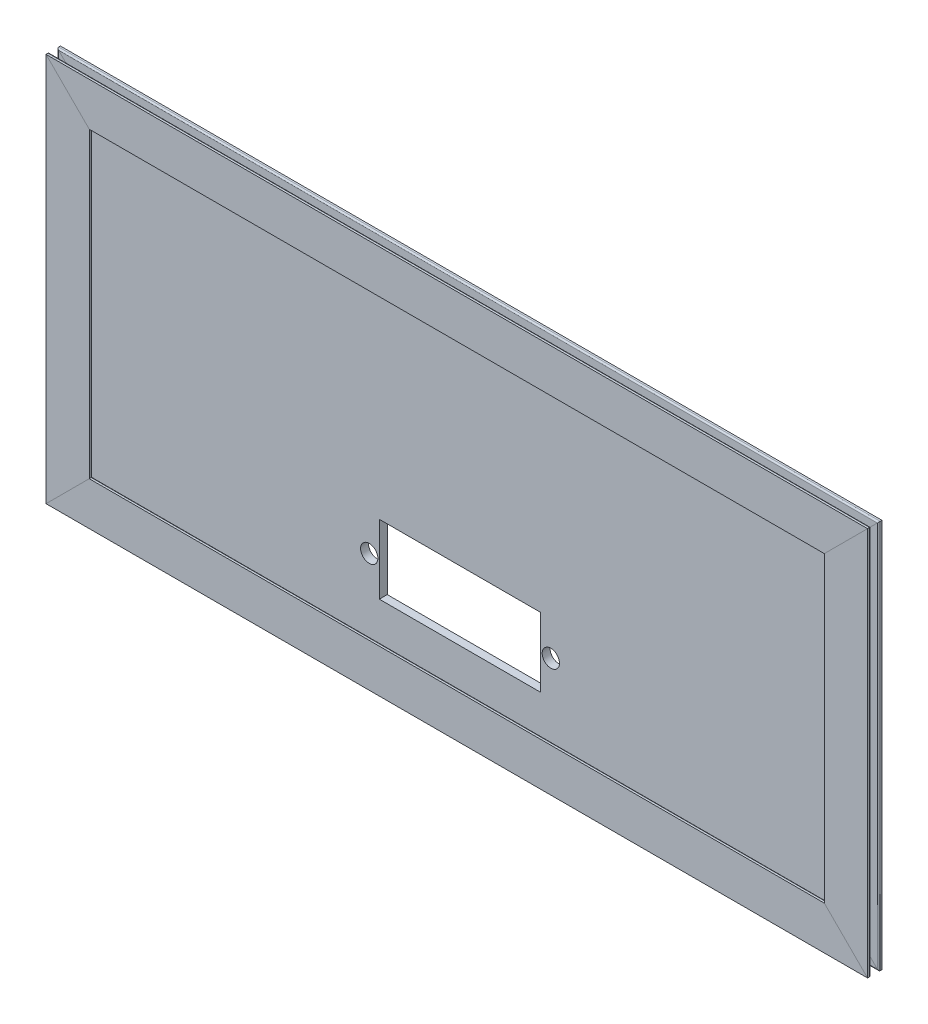
from build123d import *

# Parameters (mm, degrees)
ALUMINIUM_PROFILE_20_X_20_X_2_1_DEPTH      = 556.811388301
ALUMINIUM_PROFILE_20_X_20_X_2_1_DEPTH_BACK = 16.811388301
SKETCH1_W                                  = 6.2
SKETCH1_H                                  = 4.4
SKETCH1_ON_SEGMENT_2_W                     = 6.2
SKETCH1_ON_SEGMENT_2_H                     = 4.4
ALUMINIUM_PROFILE_20_X_20_X_2_1_2_DEPTH    = 273.622776602
SKETCH1_ON_SEGMENT_3_W                     = 6.2
SKETCH1_ON_SEGMENT_3_H                     = 4.4
ALUMINIUM_PROFILE_20_X_20_X_2_1_3_DEPTH    = 573.622776602
SKETCH1_ON_SEGMENT_4_W                     = 6.2
SKETCH1_ON_SEGMENT_4_H                     = 4.4
ALUMINIUM_PROFILE_20_X_20_X_2_1_4_DEPTH    = 273.622776602
SKETCH3_W                                  = 512
SKETCH3_H                                  = 212
BOSS_EXTRUDE1_DEPTH                        = 5.5
SKETCH4_R                                  = 6
SKETCH4_W                                  = 112
SKETCH4_H                                  = 48
CUT_EXTRUDE1_DEPTH                         = 316.452155643


with BuildPart() as part:
    # Sketch1 → Aluminium profile 20 X 20 X 2(1) (new, two sides: drawn at the far end of the back side and taken through both)
    with BuildSketch(Plane(origin=(-270, 120, 0), x_dir=(0, 1, 0), z_dir=(1, 0, 0)).offset(-ALUMINIUM_PROFILE_20_X_20_X_2_1_DEPTH_BACK)):
        with BuildLine():
            Line((4.5, 2.75), (14, 2.75))
            ThreePointArc((14, 2.75), (14.707106781, 3.042893219), (15, 3.75))
            Line((15, 3.75), (15, 5))
            Line((15, 5), (-15, 5))
            Line((-15, 5), (-15, 3.75))
            ThreePointArc((-15, 3.75), (-14.707106781, 3.042893219), (-14, 2.75))
            Line((-14, 2.75), (-4.5, 2.75))
            Line((-4.5, 2.75), (-4.5, -2.75))
            Line((-4.5, -2.75), (-14, -2.75))
            ThreePointArc((-14, -2.75), (-14.707106781, -3.042893219), (-15, -3.75))
            Line((-15, -3.75), (-15, -5))
            Line((-15, -5), (15, -5))
            Line((15, -5), (15, -3.75))
            ThreePointArc((15, -3.75), (14.707106781, -3.042893219), (14, -2.75))
            Line((14, -2.75), (4.5, -2.75))
            Line((4.5, -2.75), (4.5, 2.75))
        make_face()
        Rectangle(SKETCH1_W, SKETCH1_H, mode=Mode.SUBTRACT)
    extrude(amount=ALUMINIUM_PROFILE_20_X_20_X_2_1_DEPTH + ALUMINIUM_PROFILE_20_X_20_X_2_1_DEPTH_BACK)

    # Aluminium profile 20 X 20 X 2(1) mitre 1
    split(bisect_by=Plane(origin=(-270, 120, 0), x_dir=(-0.707106781, 0.707106781, 0), z_dir=(0.707106781, 0.707106781, 0)), keep=Keep.TOP)

    # Aluminium profile 20 X 20 X 2(1) mitre 2
    split(bisect_by=Plane(origin=(270, 120, 0), x_dir=(-0.707106781, -0.707106781, 0), z_dir=(-0.707106781, 0.707106781, 0)), keep=Keep.TOP)


with BuildPart() as body_2:
    # Sketch1 on segment 2 (carried to segment 2) → Aluminium profile 20 X 20 X 2_1 2 (new body)
    with BuildSketch(Plane(origin=(270, 136.811388301, 0), x_dir=(1, 0, 0), z_dir=(0, -1, 0))):
        with BuildLine():
            Line((4.5, 2.75), (14, 2.75))
            ThreePointArc((14, 2.75), (14.707106781, 3.042893219), (15, 3.75))
            Line((15, 3.75), (15, 5))
            Line((15, 5), (-15, 5))
            Line((-15, 5), (-15, 3.75))
            ThreePointArc((-15, 3.75), (-14.707106781, 3.042893219), (-14, 2.75))
            Line((-14, 2.75), (-4.5, 2.75))
            Line((-4.5, 2.75), (-4.5, -2.75))
            Line((-4.5, -2.75), (-14, -2.75))
            ThreePointArc((-14, -2.75), (-14.707106781, -3.042893219), (-15, -3.75))
            Line((-15, -3.75), (-15, -5))
            Line((-15, -5), (15, -5))
            Line((15, -5), (15, -3.75))
            ThreePointArc((15, -3.75), (14.707106781, -3.042893219), (14, -2.75))
            Line((14, -2.75), (4.5, -2.75))
            Line((4.5, -2.75), (4.5, 2.75))
        make_face()
        Rectangle(SKETCH1_ON_SEGMENT_2_W, SKETCH1_ON_SEGMENT_2_H, mode=Mode.SUBTRACT)
    extrude(amount=ALUMINIUM_PROFILE_20_X_20_X_2_1_2_DEPTH)

    # Aluminium profile 20 X 20 X 2_1 2 mitre
    split(bisect_by=Plane(origin=(270, -120, 0), x_dir=(-0.707106781, 0.707106781, 0), z_dir=(0.707106781, 0.707106781, 0)), keep=Keep.TOP)

    # Aluminium profile 20 X 20 X 2_1 2 mi 2
    split(bisect_by=Plane(origin=(270, 120, 0), x_dir=(0.707106781, 0.707106781, 0), z_dir=(0.707106781, -0.707106781, 0)), keep=Keep.TOP)


with BuildPart() as body_3:
    # Sketch1 on segment 3 (carried to segment 3) → Aluminium profile 20 X 20 X 2_1 3 (new body)
    with BuildSketch(Plane(origin=(286.811388301, -120, 0), x_dir=(0, -1, 0), z_dir=(-1, 0, 0))):
        with BuildLine():
            Line((4.5, 2.75), (14, 2.75))
            ThreePointArc((14, 2.75), (14.707106781, 3.042893219), (15, 3.75))
            Line((15, 3.75), (15, 5))
            Line((15, 5), (-15, 5))
            Line((-15, 5), (-15, 3.75))
            ThreePointArc((-15, 3.75), (-14.707106781, 3.042893219), (-14, 2.75))
            Line((-14, 2.75), (-4.5, 2.75))
            Line((-4.5, 2.75), (-4.5, -2.75))
            Line((-4.5, -2.75), (-14, -2.75))
            ThreePointArc((-14, -2.75), (-14.707106781, -3.042893219), (-15, -3.75))
            Line((-15, -3.75), (-15, -5))
            Line((-15, -5), (15, -5))
            Line((15, -5), (15, -3.75))
            ThreePointArc((15, -3.75), (14.707106781, -3.042893219), (14, -2.75))
            Line((14, -2.75), (4.5, -2.75))
            Line((4.5, -2.75), (4.5, 2.75))
        make_face()
        Rectangle(SKETCH1_ON_SEGMENT_3_W, SKETCH1_ON_SEGMENT_3_H, mode=Mode.SUBTRACT)
    extrude(amount=ALUMINIUM_PROFILE_20_X_20_X_2_1_3_DEPTH)

    # Aluminium profile 20 X 20 X 2_1 3 mitre
    split(bisect_by=Plane(origin=(-270, -120, 0), x_dir=(0.707106781, 0.707106781, 0), z_dir=(0.707106781, -0.707106781, 0)), keep=Keep.TOP)

    # Aluminium profile 20 X 20 X 2_1 3 mi 2
    split(bisect_by=Plane(origin=(270, -120, 0), x_dir=(0.707106781, -0.707106781, 0), z_dir=(-0.707106781, -0.707106781, 0)), keep=Keep.TOP)


with BuildPart() as body_4:
    # Sketch1 on segment 4 (carried to segment 4) → Aluminium profile 20 X 20 X 2_1 4 (new body)
    with BuildSketch(Plane(origin=(-270, -136.811388301, 0), x_dir=(-1, 0, 0), z_dir=(0, 1, 0))):
        with BuildLine():
            Line((4.5, 2.75), (14, 2.75))
            ThreePointArc((14, 2.75), (14.707106781, 3.042893219), (15, 3.75))
            Line((15, 3.75), (15, 5))
            Line((15, 5), (-15, 5))
            Line((-15, 5), (-15, 3.75))
            ThreePointArc((-15, 3.75), (-14.707106781, 3.042893219), (-14, 2.75))
            Line((-14, 2.75), (-4.5, 2.75))
            Line((-4.5, 2.75), (-4.5, -2.75))
            Line((-4.5, -2.75), (-14, -2.75))
            ThreePointArc((-14, -2.75), (-14.707106781, -3.042893219), (-15, -3.75))
            Line((-15, -3.75), (-15, -5))
            Line((-15, -5), (15, -5))
            Line((15, -5), (15, -3.75))
            ThreePointArc((15, -3.75), (14.707106781, -3.042893219), (14, -2.75))
            Line((14, -2.75), (4.5, -2.75))
            Line((4.5, -2.75), (4.5, 2.75))
        make_face()
        Rectangle(SKETCH1_ON_SEGMENT_4_W, SKETCH1_ON_SEGMENT_4_H, mode=Mode.SUBTRACT)
    extrude(amount=ALUMINIUM_PROFILE_20_X_20_X_2_1_4_DEPTH)

    # Aluminium profile 20 X 20 X 2_1 4 mitre
    split(bisect_by=Plane(origin=(-270, -120, 0), x_dir=(-0.707106781, -0.707106781, 0), z_dir=(-0.707106781, 0.707106781, 0)), keep=Keep.TOP)

    # Aluminium profile 20 X 20 X 2_1 4 mi 2
    split(bisect_by=Plane(origin=(-270, 120, 0), x_dir=(0.707106781, -0.707106781, 0), z_dir=(-0.707106781, -0.707106781, 0)), keep=Keep.TOP)


with BuildPart() as body_5:
    # Sketch3 → Boss-Extrude1 (new body)
    with BuildSketch(Plane.XY.offset(-2.75)):
        Rectangle(SKETCH3_W, SKETCH3_H)
    extrude(amount=BOSS_EXTRUDE1_DEPTH)

    # Sketch4 → Cut-Extrude1 (cut, through all)
    with BuildSketch(Plane(origin=(0, 0, -2.75), x_dir=(-1, 0, 0), z_dir=(0, 0, -1))):
        with Locations((-63, -55)):
            Circle(SKETCH4_R)
        with Locations((63, -55)):
            Circle(SKETCH4_R)
        with Locations((0, -55)):
            Rectangle(SKETCH4_W, SKETCH4_H)
    extrude(amount=-CUT_EXTRUDE1_DEPTH, mode=Mode.SUBTRACT)


solid = Compound([part.part, body_2.part, body_3.part, body_4.part, body_5.part])
